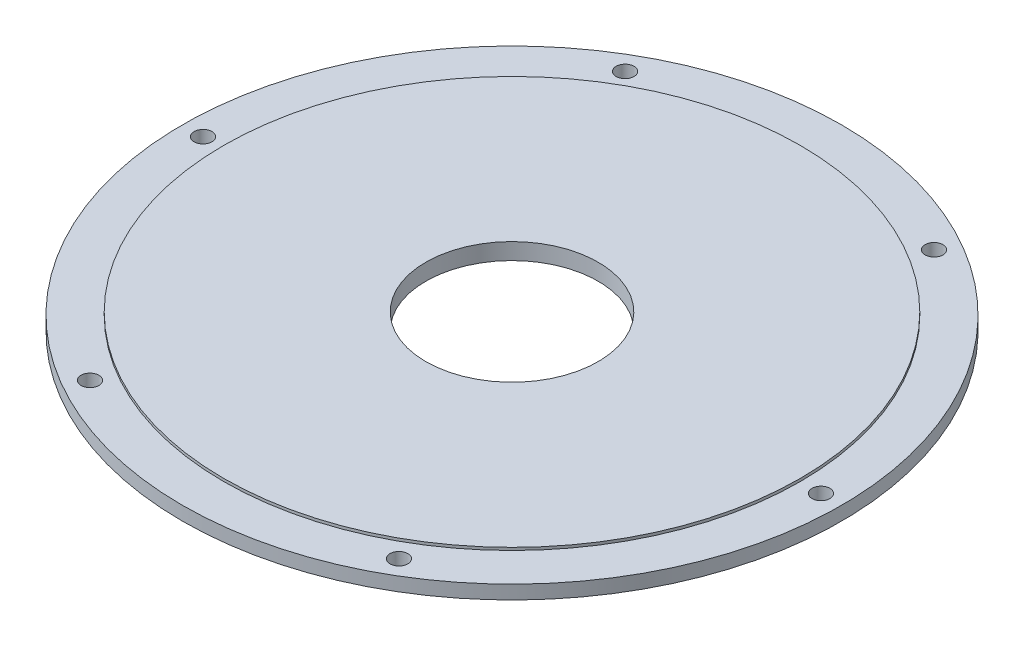
from build123d import *

# Parameters (mm, degrees)
SKETCH1_R                  = 240
SKETCH1_R_2                = 62.75
BOSS_EXTRUDE1_DEPTH        = 6
F_13_0_13_DIAMETER_HOLE1_D = 13
SKETCH4_OUTSIDE_W          = 617.786
SKETCH4_OUTSIDE_H          = 617.786
SKETCH4_OUTSIDE_R          = 210
CUT_EXTRUDE1_DEPTH         = 2


with BuildPart() as part:
    # Sketch1 → Boss-Extrude1 (new, symmetric)
    with BuildSketch(Plane(origin=(0, 0, 0), x_dir=(1, 0, 0), z_dir=(0, 1, 0))):
        with Locations(Location((0, 0, 0), (0, 0, 270))):
            Circle(SKETCH1_R)
        with Locations(Location((0, 0, 0), (0, 0, 270))):
            Circle(SKETCH1_R_2, mode=Mode.SUBTRACT)
    extrude(amount=BOSS_EXTRUDE1_DEPTH, both=True)

    # Ø13.0 (13) Diameter Hole1 (through all)
    with Locations(Plane(origin=(0, 6, 0), x_dir=(1, 0, 0), z_dir=(0, 1, 0))):
        with Locations((112.5, -194.855715851), (-112.5, -194.855715851), (-225, 0), (-112.5, 194.855715851), (112.5, 194.855715851), (225, 0)):
            Hole(F_13_0_13_DIAMETER_HOLE1_D / 2)

    # Sketch4 outside → Cut-Extrude1 (cut)
    with BuildSketch(Plane(origin=(0, 6, 0), x_dir=(1, 0, 0), z_dir=(0, 1, 0))):
        Rectangle(SKETCH4_OUTSIDE_W, SKETCH4_OUTSIDE_H)
        with Locations(Location((0, 0, 0), (0, 0, 270))):
            Circle(SKETCH4_OUTSIDE_R, mode=Mode.SUBTRACT)
    extrude(amount=-CUT_EXTRUDE1_DEPTH, mode=Mode.SUBTRACT)


solid = part.part
